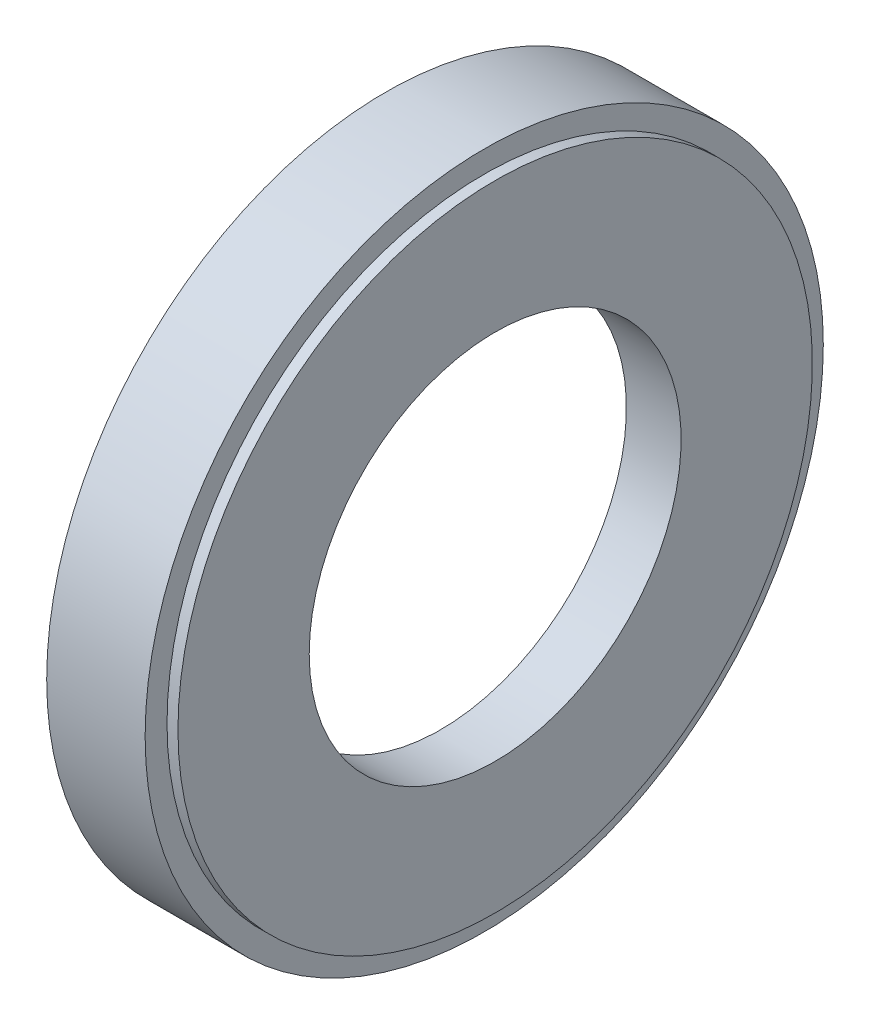
from build123d import *


with BuildPart() as part:
    # 草图1 → 旋转1 (revolve)
    with BuildSketch(Plane.XY, mode=Mode.PRIVATE) as revolve_1_sk:
        Polygon((-1.646669205, 17), (3.353330795, 17), (3.353330795, 29), (2.353330795, 29), (2.353330795, 31), (-6.646669205, 31), (-6.646669205, 29), (-1.646669205, 29), align=None)
    revolve(revolve_1_sk.sketch.rotate(Axis((0, 0, 0), (1, 0, 0)), 90), axis=Axis((0, 0, 0), (1, 0, 0)))


solid = part.part
